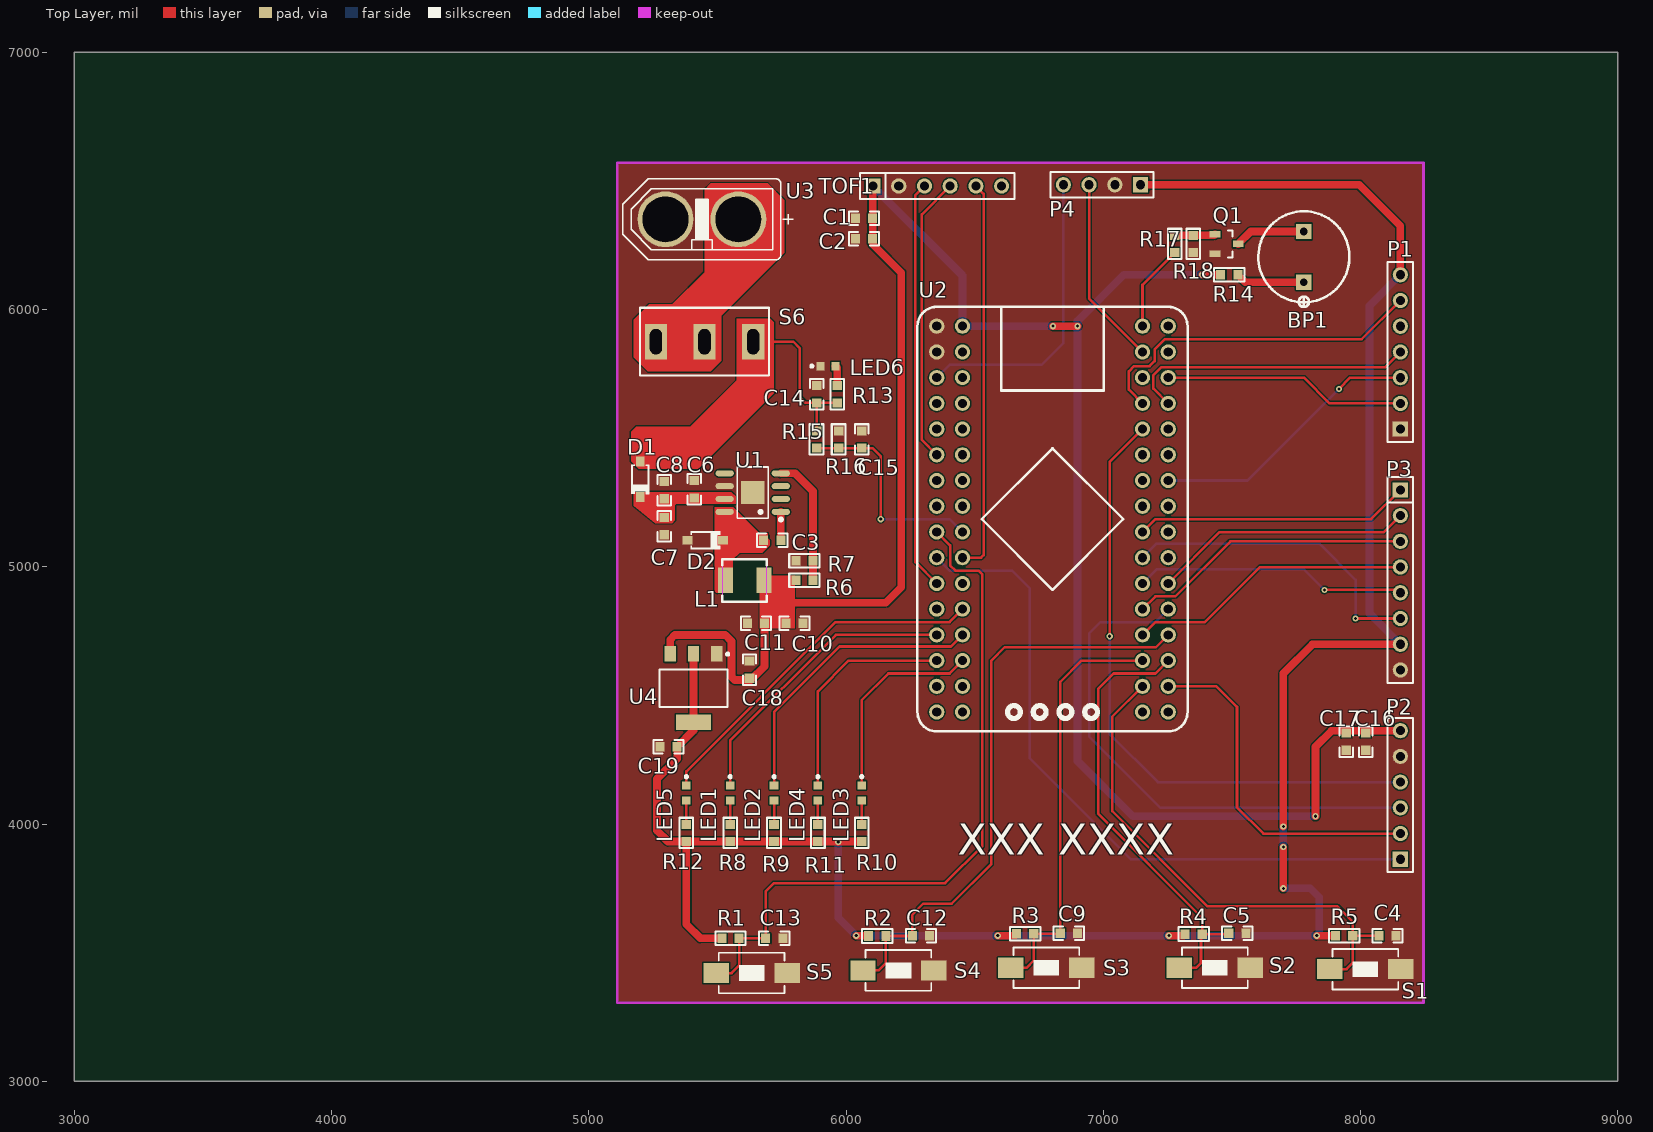
[diagram p0: Top Layer view]
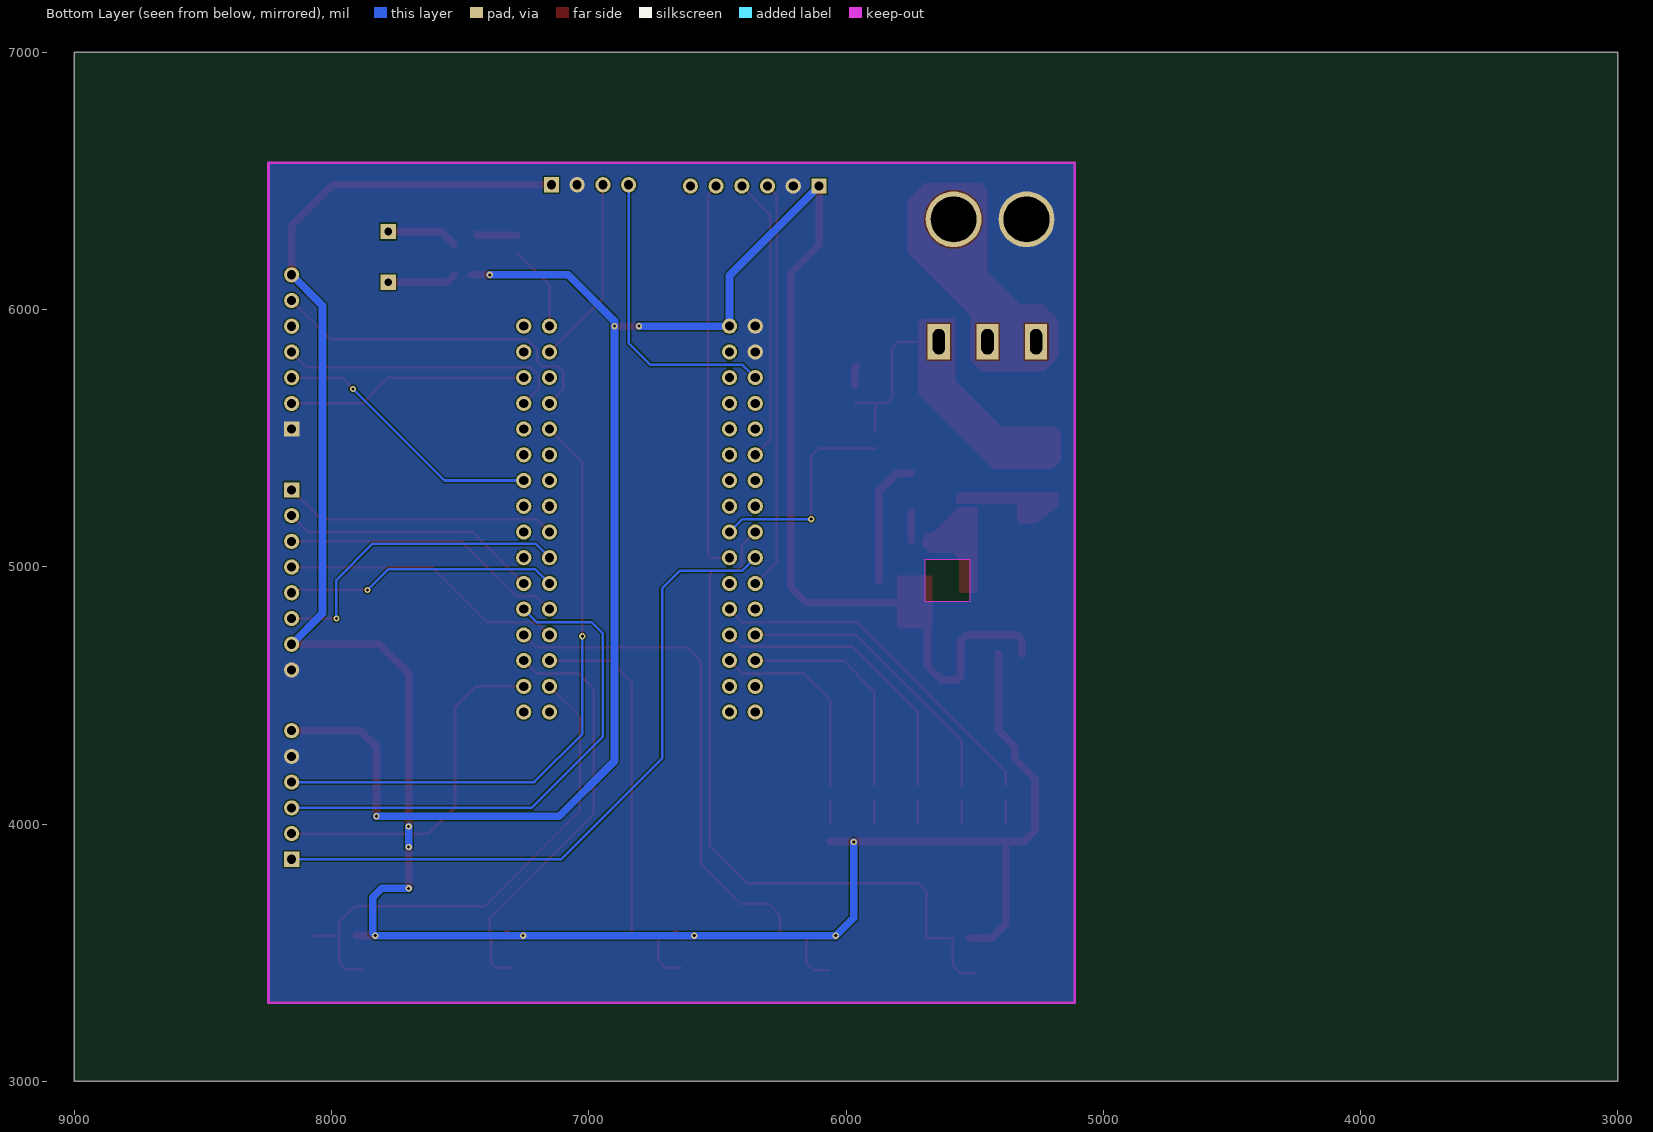
[diagram p1: Bottom Layer view, seen from below]
# Altium PCB MISC75116.pcbdoc
Units mil, origin at the board's own origin, x right, y up, seen from the top; angles counter-clockwise.
Board outline 6000 x 4000 mil, 2 copper layers (Top Layer, Bottom Layer); 63 components, 49 nets, 220 pads, 17 vias.

## Layer stack, top to bottom (the 12.6 mil dielectric is the usual default, probably not edited)
Top Solder Mask Layer: solder mask 0.4, Solder Resist, Dk 3.5
Top Layer: signal copper 1.4
Dielectric 1: surface 12.6, FR-4, Dk 4.8
Bottom Layer: signal copper 1.4
Bottom Solder Mask Layer: solder mask 0.4, Solder Resist, Dk 3.5

## Board outline
3000,7000 3000,3000 9000,3000 9000,7000

## Design rules (kind name [scope] priority, off if disabled: settings)
BoardOutlineClearance Clearance_1 [All] p2: genericclearance=5 ignorepadtopadclearanceinfootprint=FALSE except(0: Arc-SplitContinuation Track-SplitContinuation SMDPad-SplitContinuation THPad-SplitContinuation Via-SplitContinuation Fill-SplitContinuation Region-SplitContinuation Poly-SplitContinuation Text-SplitContinuation Hole-SplitContinuation; 5: Arc-OutlineEdge Track-OutlineEdge SMDPad-OutlineEdge THPad-OutlineEdge Via-OutlineEdge Fill-OutlineEdge Region-OutlineEdge Poly-OutlineEdge Text-OutlineEdge Hole-OutlineEdge SMDPad-CutoutEdge THPad-CutoutEdge Poly-CutoutEdge; 6: Via-CutoutEdge Fill-CutoutEdge Region-CutoutEdge Text-CutoutEdge; 6.9: Hole-CutoutEdge; 11.8: Arc-CutoutEdge Track-CutoutEdge)
Clearance [All] p1: gap=5 ignorepadtopadclearanceinfootprint=FALSE
DiffPairsRouting [All] p1: maxlimit=10 minlimit=6 mostfreqgap=6 toplayer_minwidth=15 toplayer_prefwidth=15 toplayer_maxwidth=15 toplayer_mingap=10 toplayer_prefgap=10 toplayer_maxgap=10 bottomlayer_minwidth=15 bottomlayer_prefwidth=15 bottomlayer_maxwidth=15 bottomlayer_mingap=10 bottomlayer_prefgap=10 bottomlayer_maxgap=10 maxuncoupledlength=10
HoleToHoleClearance ComponentClearance [All] p1: gap=10 allowstackedmicrovias=TRUE
Length netLength [All] p1: minlimit=0 maxlimit=0
MatchedLengths netLengthTolerance [All] p1: tolerance=1000
PlaneConnect [All] p1: planeconnectstyle=Direct reliefexpansion=20 reliefentries=4 reliefconductorwidth=10 reliefairgap=10
PolygonConnect [(InNet('GND'))] p1: connectstyle=Direct reliefconductorwidth=10 reliefentries=4 polygonreliefangle="90 Angle" airgapwidth=10 via.connectstyle=Relief via.reliefconductorwidth=10 via.reliefentries=4 via.polygonreliefangle="90 Angle" via.airgapwidth=10
RoutingVias [All] p1: holewidth=28 width=50 viastyle="Through Hole" minholewidth=2 minwidth=2 maxholewidth=28 maxwidth=50
SolderMaskExpansion [All] p1: expansion=4 istentingtop=FALSE
Width [All] p1: maxlimit=10 minlimit=10 preferedwidth=10 toplayer_minwidth=10 toplayer_maxwidth=200 toplayer_prefwidth=10 bottomlayer_minwidth=10 bottomlayer_maxwidth=200 bottomlayer_prefwidth=10
1 further rules are at their usual default settings.

## Components (designator, comment, footprint, x,y, rotation, side; value= is the part's Value field where it differs from the comment)
BP1 "Buzzer" 5*10fengmiqi 7780,6205 r90 top
C1 "10uF" CAPC1608[0603]S-N 6070.16,6354.81 r0 top
C2 "0.1uF" CAPC1608[0603]S-N 6070.16,6275.25 r0 top
C3 "100nF" CAPC1608[0603]S-N 5713.43,5103.06 r180 top
C4 "10uF" CAPC1608[0603]S-N 8105,3565 r0 top
C5 "10uF" CAPC1608[0603]S-N 7521.45,3575.86 r0 top
C6 "0.1uF" CAPC1608[0603]S-N 5409.96,5301.52 r270 top
C7 "4.7uF" CAPC1608[0603]S-N 5293.43,5158.06 r90 top
C8 "4.7uF" CAPC1608[0603]S-N 5293.43,5298.06 r270 top
C9 "10uF" CAPC1608[0603]S-N 6866.45,3575.86 r0 top
C10 "100uF" CAPC1608[0603]S-N 5800,4780 r0 top
C11 "0.1uF" CAPC1608[0603]S-N 5650,4780 r0 top
C12 "10uF" CAPC1608[0603]S-N 6291.45,3565.86 r0 top
C13 "10uF" CAPC1608[0603]S-N 5721.16,3555.57 r0 top
C14 "1000uF  25V" CAPC1608[0603]S-N 5885.73,5670.69 r90 top
C15 "100nF 50V X7R" CAPC1608[0603]S-N 6060.57,5495 r90 top
C16 "0.1uF ±10% 25V" CAPC1608[0603]S-N 8020,4320 r270 top
C17 "10uF ±10% 50V" CAPC1608[0603]S-N 7945,4320 r270 top
C18 "1uF" CAPC1608[0603]S-N 5625,4600 r270 top
C19 "1uF" CAPC1608[0603]S-N 5310,4300 r0 top
D1 "SS54" SOD-123-L 5200,5340 r270 top
D2 "SS54" SOD-123-L 5453.43,5103.06 r0 top
L1 "4.7uH 2.5A" "0402 TPC 4*4*2" 5573.43,4893.06 r270 top
LED1 "LED" LEDC1608(0603) 5549.84,4120.74 r270 top
LED2 "LED" LEDC1608(0603) 5720.31,4120.74 r270 top
LED3 "LED" LEDC1608(0603) 6061.24,4120.74 r270 top
LED4 "LED" LEDC1608(0603) 5890.77,4120.74 r270 top
LED5 "LED" LEDC1608(0603) 5379.37,4120.74 r270 top
LED6 "LED" LEDC1608(0603) 5930,5780 r0 top
P1 "Header 7" HDR1X7 8155,5535 r90 top
P2 "Gyroscope" HDR1X6 8155,3862.78 r90 top
P3 "Header  1X8" HDR1X8 8155,5298.89 r270 top
P4 "Header-D-M 1x4P" HDR1X4 7145,6485 r180 top
Q1 "S8050" SOT-23 7479.78,6255.03 r0 top
R1 "1K" RESC1608[0603]S-N 5551.16,3555.57 r180 top
R2 "1K" RESC1608[0603]S-N 6121.45,3564.61 r180 top
R3 "1K" RESC1608[0603]S-N 6696.45,3573.36 r180 top
R4 "1K" RESC1608[0603]S-N 7351.45,3572.11 r180 top
R5 "1K" RESC1608[0603]S-N 7936.45,3565.86 r180 top
R6 "10K" RESC1608[0603]S-N 5838.43,4948.06 r180 top
R7 "3K" RESC1608[0603]S-N 5838.43,5023.06 r180 top
R8 "10K" RESC1608[0603]S-N 5549.84,3965.27 r90 top
R9 "10K" RESC1608[0603]S-N 5720.31,3965.27 r90 top
R10 "10K" RESC1608[0603]S-N 6061.24,3965.27 r90 top
R11 "10K" RESC1608[0603]S-N 5890.77,3965.27 r90 top
R12 "10K" RESC1608[0603]S-N 5379.37,3965.27 r90 top
R13 "1K" RESC1608[0603]S-N 5965.87,5670.69 r90 top
R14 "10R ±1%" RESC1608[0603]S-N 7490,6135 r0 top
R15 "10K ±1%" RESC1608[0603]S-N 5885.57,5495 r270 top
R16 "1K ±1%" RESC1608[0603]S-N 5971.15,5495 r90 top
R17 "4.7K ±1%" RESC1608[0603]S-N 7278.09,6255.03 r90 top
R18 "10K ±1%" RESC1608[0603]S-N 7350,6255 r270 top
S1 "KEY" anjiantiepiankaiguan 8021.45,3435.86 r0 top
S2 "KEY" anjiantiepiankaiguan 7436.45,3440.86 r0 top
S3 "KEY" anjiantiepiankaiguan 6781.45,3440.86 r0 top
S4 "KEY" anjiantiepiankaiguan 6206.45,3430.86 r0 top
S5 "KEY" anjiantiepiankaiguan 5636.16,3420.57 r0 top
S6 "SW" SS12D10 5450,5875 r0 top
TOF1 "Ranging module" HDR1X6 6105,6480 r0 top
U1 "TPS5450" 5450 5603.43,5283.06 r90 top
U2 "STC32G12K128" STC16F40K128_CoreBoard 6802.78,5185.25 r0 top
U3 "XT60-F" XT60 5455.61,6421.45 r0 top
U4 "LM1117" "LM1117 - duplicate" 5417.17,4518.45 r180 top

## Footprints (in the part's own frame and the unit in brackets; to place one, negate y for a bottom-side part, rotate by r counter-clockwise, add the part's x,y. Pads: shape width x height; smd on the part's side, far side on the other; paste and mask are expansions set on the pad)
5*10fengmiqi [mil]
  rect 60x60 hole 30: 1(-98.43,0) 2(98.43,0)
  silkscreen extent -195,-177 177,177
"0402 TPC 4*4*2" [mm]
  rect 2.5x1.5 smd: 1(-1.371,-1.076) 2(-1.371,2.724)
  silkscreen extent -3.47,-1.38 0.73,3.02
5450 [mm]
  oval 0.6x1.8 smd paste+0 mask+0.051: 1(-1.77,-3.638) 2(-0.5,-3.638) 3(0.77,-3.638) 4(2.04,-3.638) 5(2.04,1.907) 6(0.77,1.907) 7(-0.5,1.907) 8(-1.77,1.907)
  rect 2.29x2.29 smd paste+0 mask+0.051: 9(0.135,-0.866)
  silkscreen extent -2.67,-3.79 2.66,0.66
anjiantiepiankaiguan [mm]
  rect 2.5x2 smd: 1(3.429,0) 2(-3.571,0)
  silkscreen extent -3.32,-2 3.18,2
CAPC1608[0603]S-N [mm]
  rect 0.9x0.95 smd: 1(-0.85,0) 2(0.85,0)
  silkscreen extent -1.5,-0.66 1.5,0.66
HDR1X4 [mm]
  rect 1.5x1.5 hole 0.9: 1(0,0)
  round 1.5 hole 0.9: 2(2.54,0) 3(5.08,0) 4(7.62,0)
  silkscreen extent -1.27,-1.27 8.89,1.27
HDR1X6 [mm]
  rect 1.5x1.5 hole 0.9: 1(0,0)
  round 1.5 hole 0.9: 2(2.54,0) 3(5.08,0) 4(7.62,0) 5(10.16,0) 6(12.7,0)
  silkscreen extent -1.27,-1.27 13.97,1.27
HDR1X7 [mm]
  rect 1.5x1.5 hole 0.9: 1(0,0)
  round 1.5 hole 0.9: 2(2.54,0) 3(5.08,0) 4(7.62,0) 5(10.16,0) 6(12.7,0) 7(15.24,0)
  silkscreen extent -1.27,-1.27 16.51,1.27
HDR1X8 [mm]
  rect 1.5x1.5 hole 0.9: 1(0,0)
  round 1.5 hole 0.9: 2(2.54,0) 3(5.08,0) 4(7.62,0) 5(10.16,0) 6(12.7,0) 7(15.24,0) 8(17.78,0)
  silkscreen extent -1.27,-1.27 19.05,1.27
LEDC1608(0603) [mm]
  rect 0.8x0.85 smd: A(0.75,0) C(-0.75,0)
  silkscreen extent -1.72,-0.12 -1.48,0.12
"LM1117 - duplicate" [mm]
  rect 1.1x1.55 smd: 1(-2.046,-3.629) 2(0.254,-3.629) 3(2.554,-3.629)
  rect 3.45x1.55 smd: 4(0.254,3.121)
  silkscreen extent -3.25,-3.73 3.6,1.6
RESC1608[0603]S-N [mm]
  rect 0.9x0.95 smd: 1(-0.85,0) 2(0.85,0)
  silkscreen extent -1.5,-0.67 1.5,0.67
SOD-123-L [mm]
  rect 1x0.85 smd: A(-1.75,0) K(1.75,0)
  silkscreen extent -1.45,-0.9 1.47,0.9
SOT-23 [mm]
  rect 1.05x0.65 smd: 1(-1.15,0.95) 2(-1.15,-0.95) 3(1.15,0)
  silkscreen extent 0.13,-1.35 0.58,1.35
SS12D10 [mm]
  rect 2.2x3.5 hole 1.2 slot 2.5 at 90 deg paste+0 mask+0.07: 1(-4.8,0) 2(0,0) 3(4.8,0)
  silkscreen extent -6.35,-3.35 6.35,3.35
STC16F40K128_CoreBoard [mm]
  round 1.5 hole 0.9: 1(-11.43,19.05) 2(-8.89,19.05) 3(-11.43,16.51) 4(-8.89,16.51) 5(-11.43,13.97) 6(-8.89,13.97) 7(-11.43,11.43) 8(-8.89,11.43) 9(-11.43,8.89) 10(-8.89,8.89) 11(-11.43,6.35) 12(-8.89,6.35) 13(-11.43,3.81) 14(-8.89,3.81) 15(-11.43,1.27) 16(-8.89,1.27) 17(-11.43,-1.27) 18(-8.89,-1.27) 19(-11.43,-3.81) 20(-8.89,-3.81) 21(-11.43,-6.35) 22(-8.89,-6.35) 23(-11.43,-8.89) 24(-8.89,-8.89) 25(-11.43,-11.43) 26(-8.89,-11.43) 27(-11.43,-13.97) 28(-8.89,-13.97) 29(-11.43,-16.51) 30(-8.89,-16.51) 31(-11.43,-19.05) 32(-8.89,-19.05) 33(8.89,-19.05) 34(11.43,-19.05) 35(8.89,-16.51) 36(11.43,-16.51) 37(8.89,-13.97) 38(11.43,-13.97) 39(8.89,-11.43) 40(11.43,-11.43) 41(8.89,-8.89) 42(11.43,-8.89) 43(8.89,-6.35) 44(11.43,-6.35) 45(8.89,-3.81) 46(11.43,-3.81) 47(8.89,-1.27) 48(11.43,-1.27) 49(8.89,1.27) 50(11.43,1.27) 51(8.89,3.81) 52(11.43,3.81) 53(8.89,6.35) 54(11.43,6.35) 55(8.89,8.89) 56(11.43,8.89) 57(8.89,11.43) 58(11.43,11.43) 59(8.89,13.97) 60(11.43,13.97) 61(8.89,16.51) 62(11.43,16.51) 63(8.89,19.05) 64(11.43,19.05)
  silkscreen extent -13.33,-20.95 13.33,20.95
XT60 [mil]
  round 217.16 hole 177.16 slot 177.36 at 0 deg paste+0 mask+2: ""(-157.43,-70.62) ""(126.03,-70.62)
  silkscreen extent -323,-228 339,87

## Via types
v1: diameter 24.02, hole 12, Top Layer to Bottom Layer, 17 vias

## Nets (pads, with @x,y where several pads share a name; then routed paths per layer and width w, separated by ;. In a path a pad name is that pad's centre, name@x,y a point inside that pad or via, vN(x,y) a via of type N, cw(c..) or ccw(c..) an arc to the next point about the centre after c; other vN are vias at no path point)
0.2: P1.3 U2.52 | length 1067.8
  Top Layer w10: v1(7916.35,5691.35) 7960,5735 P1.3
  Bottom Layer w10: U2.52 7560.25,5335.25 v1(7916.35,5691.35)
0.3: P1.4 U2.58 | length 1131
  Top Layer w10: U2.58 7195,5693.03 7195,5745 7225,5775 8095,5775 P1.4
1.0: P4.3 U2.61 | length 735.8
  Top Layer w10: P4.3 6945,6043.03 U2.61
1.1: P4.4 U2.5 | length 1163
  Bottom Layer w10: U2.5 6402.53,5785 6760,5785 6845,5870 P4.4
3V3: C19.2 P1.7 P3.7 P4.1 R1.2 R2.2 R3.2 R4.2 R5.2 R8.1 R9.1 R10.1 R11.1 R12.1 U4.2 U4.4 | length 8936.2
  Top Layer w30: U4.2 U4.4 5407.17,4363.71 C19.2 5343.46,4253.46 5265,4175 5265,3975 5308.19,3931.81 R12.1 ; R1.2 5434.43,3555.57 5379.37,3610.63 R12.1 ; v1(6040,3565.86) 6086.73,3565.86 R2.2 ; R10.1 5971.81,3931.81 v1(5970,3930) 5968.19,3931.81 R11.1 R9.1 R8.1 R12.1 ; v1(6590,3565.86) 6655.48,3565.86 R3.2 ; P4.1 7995,6485 8155,6325 P1.7 ; v1(7255,3565.86) 7311.73,3565.86 R4.2 ; v1(7700,3750) v1(7700,3910) ; v1(7700,3990) 7700,4585 7813.89,4698.89 P3.7 ; v1(7830,3565.86) R5.2
  Bottom Layer w30: v1(5970,3930) 5970,3635.86 v1(6040,3565.86) v1(6590,3565.86) v1(7255,3565.86) v1(7830,3565.86) 7840,3575.86 7840,3715 7805,3750 v1(7700,3750) ; v1(7700,3910) v1(7700,3990) ; P3.7 8035,4818.89 8035,6015 P1.7
4: P1.6 U2.57 | length 1342.3
  Top Layer w10: U2.57 7099.52,5688.51 7099.52,5759.52 7120,5780 7180,5780 7200,5800 7200,5845 7240,5885 8005,5885 P1.6
5: P1.2 U2.60 | length 943.7
  Top Layer w10: U2.60 7779.75,5735.25 7880,5635 P1.2
5V: C1.2 C2.2 C10.1 C11.2 C16.1 C17.1 C18.2 L1.2 P2.6 R6.2 R14.1 TOF1.1 U2.2 U4.3 | length 7965.5
  Top Layer w30: U4.3 5316.62,4716.62 5335,4735 5530,4735 5555,4710 5555,4572.08 5567.08,4560 5630,4560 5683.46,4613.46 C11.2 ; 5770,4860 6155,4860 6215,4920 6215,6142.84 6103.62,6254.21 C2.2 C1.2 6103.62,6478.62 TOF1.1 ; v1(6805,5935.25) v1(6900,5935.25) ; v1(7385,6135) R14.1 ; v1(7825,4030) 7825,4300 7887.78,4362.78 P2.6
  Bottom Layer w30: TOF1.1 6452.78,6132.22 U2.2 v1(6805,5935.25) ; v1(7385,6135) 7080,6135 6900,5955 v1(6900,5935.25) 6900,4245 7115,4030 v1(7825,4030)
12V: C14.1 D1.A R13.1 R15.1 S6.3 | length 645.5
  Top Layer w10: S6.3 5795,5875 5820,5850 5820,5660 5842.78,5637.22 C14.1 ; R15.1 5885.73,5528.62 C14.1 ; R13.1 C14.1
17: C15.1 R15.2 R16.1 U2.18 | length 845.9
  Top Layer w10: R15.2 R16.1 C15.1 6103.46,5461.54 6135,5430 v1(6135,5185)
  Bottom Layer w10: v1(6135,5185) 6403.03,5185 U2.18
20: P3.4 U2.39 | length 1111.4
  Top Layer w10: U2.39 7202.53,4785 7395,4785 7608.89,4998.89 P3.4
21: P3.3 U2.41 | length 1111.4
  Top Layer w10: U2.41 7202.53,4885 7280,4885 7493.89,5098.89 P3.3
22: P3.2 U2.44 | length 1011.4
  Top Layer w10: U2.44 7452.53,5135 8091.11,5135 P3.2
23: P3.5 U2.43 | length 1062.6
  Top Layer w10: v1(7860,4910) 8143.89,4910 P3.5
  Bottom Layer w10: U2.43 7207.53,4990 7780,4990 v1(7860,4910)
25: P3.6 U2.45 | length 1233.3
  Top Layer w10: v1(7981.11,4798.89) P3.6
  Bottom Layer w10: U2.45 7207.53,5090 7840,5090 7981.11,4948.89 v1(7981.11,4798.89)
27: P3.1 U2.47 | length 1070
  Top Layer w10: U2.47 7202.53,5185 8041.11,5185 P3.1
30: LED1.C U2.25 | length 1147.5
  Top Layer w10: LED1.C 5549.84,4324.84 5960.25,4735.25 U2.25
31: LED2.C U2.26 | length 1141.8
  Top Layer w10: LED2.C 5720.31,4435.31 5975,4690 6407.53,4690 U2.26
32: LED3.C U2.28 | length 786.3
  Top Layer w10: LED3.C 6061.24,4481.24 6165,4585 6402.53,4585 U2.28
33: LED4.C U2.27 | length 877
  Top Layer w10: LED4.C 5890.77,4515.77 6010.25,4635.25 U2.27
40: P2.1 U2.19 | length 2674.5
  Bottom Layer w10: U2.19 6403.03,4985 6645,4985 6715,4915 6715,4255 7107.22,3862.78 P2.1
41: P2.2 U2.36 | length 1367.8
  Top Layer w10: U2.36 7439.75,4535.25 7520,4455 7520,4065 7622.22,3962.78 P2.2
42: P2.3 U2.42 | length 2072.1
  Bottom Layer w10: U2.42 7202.53,4785 6990,4785 6945,4740 6945,4340 7222.22,4062.78 P2.3
43: P2.4 U2.55 | length 2445.7
  Top Layer w10: v1(7025,4730) 7025,5407.47 U2.55
  Bottom Layer w10: v1(7025,4730) 7025,4350 7212.22,4162.78 P2.4
46: R17.1 U2.63 | length 338.2
  Top Layer w10: U2.63 7152.78,6096.25 R17.1
47: TOF1.5 U2.20 | length 1533.7
  Top Layer w10: U2.20 6525.25,5035.25 6535,5045 6535,6450 TOF1.5
63: TOF1.4 U2.11 | length 1114.2
  Top Layer w10: U2.11 6295,5493.03 6295,6370 TOF1.4
65: TOF1.3 U2.21 | length 1593.5
  Top Layer w10: TOF1.3 6270,6445 6270,5018.03 U2.21
66: LED5.C U2.24 | length 1388.8
  Top Layer w10: LED5.C 5379.37,4204.37 5960,4785 6402.53,4785 U2.24
70: C4.1 R5.1 S1.2 U2.35 | length 2008.2
  Top Layer w10: U2.35 7035,4417.47 7035,4050 7405,3680 7910,3680 7969.91,3620.09 R5.1 ; S1.2 7945.86,3435.86 7969.91,3459.91 R5.1 ; C4.1 8070.68,3565.86 R5.1
71: C5.1 R4.1 S2.2 U2.38 | length 1749.9
  Top Layer w10: U2.38 7202.53,4585 7040,4585 6980,4525 6980,4040 7384.91,3635.09 R4.1 ; S2.2 7360.86,3440.86 7380,3460 7380,3567.2 R4.1 ; C5.1 7484.23,3572.11 R4.1
72: C9.1 R3.1 S3.2 U2.37 | length 1639.6
  Top Layer w10: S3.2 6700.86,3440.86 6729.91,3469.91 R3.1 6830.48,3573.36 C9.1 6832.98,4552.98 6915.25,4635.25 U2.37
73: C12.1 R2.1 S4.2 U2.40 | length 2299.4
  Top Layer w10: S4.2 6125.86,3430.86 6154.91,3459.91 R2.1 6256.73,3564.61 C12.1 6257.98,3647.98 6300,3690 6410,3690 6565,3845 6565,4635 6617.07,4687.07 7204.6,4687.07 U2.40
GND: C1.1 C2.1 C4.2 C5.2 C6.1 C7.1 C8.1 C9.2 C10.2 C11.1 C12.2 C13.2 C14.2 C15.2 C16.2 C17.2 C18.1 C19.1 D2.A LED6.C P1.1 P2.5 P3.8 P4.2 Q1.2 R7.2 R16.2 R18.2 S1.1 S2.1 S3.1 S4.1 S5.1 TOF1.2 U1.6 U1.9 U2.1 U2.3 U3.@5298.18,6350.83 U4.1
NetBP1_1: BP1.1 R14.2 | length 268.3
  Top Layer w30: R14.2 7551.89,6106.57 BP1.1
NetBP1_2: BP1.2 Q1.3 | length 275
  Top Layer w30: Q1.3 7573.46,6303.43 BP1.2
NetC3_1: C3.1 U1.1 | length 110.4
  Top Layer w30: U1.1 5746.67,5103.28 C3.1
NetC3_2: C3.2 D2.K L1.1 U1.8
NetC6_2: C6.2 C7.2 C8.2 D1.K U1.7
NetLED1_A: LED1.A R8.2 | length 92.5
  Top Layer w10: R8.2 LED1.A
NetLED2_A: LED2.A R9.2 | length 92.5
  Top Layer w10: R9.2 LED2.A
NetLED3_A: LED3.A R10.2 | length 92.5
  Top Layer w10: R10.2 LED3.A
NetLED4_A: LED4.A R11.2 | length 92.5
  Top Layer w10: R11.2 LED4.A
NetLED5_A: LED5.A R12.2 | length 92.5
  Top Layer w10: R12.2 LED5.A
NetLED6_A: LED6.A R13.2 | length 78.5
  Top Layer w30: LED6.A 5965.87,5773.66 R13.2
NetQ1_1: Q1.1 R17.2 R18.1 | length 158
  Top Layer w30: R17.2 R18.1 7430.57,6288.49 Q1.1
NetR6_1: R6.1 R7.1 U1.4 | length 499.4
  Top Layer w30: U1.4 5801.64,5363.36 5871.89,5293.11 R7.1 R6.1
NetS6_1: S6.1 S6.2 U3.@5581.64,6350.83
RST: C13.1 R1.1 S5.2 U2.17 | length 2754.4
  Top Layer w10: S5.2 5555.57,3420.57 5584.62,3449.62 R1.1 C13.1 5687.69,3737.69 5720,3770 6385,3770 6530,3915 6530,4970.11 6515.11,4985 6425,4985 6405,5005 6405,5083.03 U2.17
pads on no net: P1.5 TOF1.6 U1.2 U1.3 U1.5 U2.4 U2.6 U2.7 U2.8 U2.9 U2.10 U2.12 U2.13 U2.14 U2.15 U2.16 U2.22 U2.23 U2.29 U2.30 U2.31 U2.32 U2.33 U2.34 U2.46 U2.48 U2.49 U2.50 U2.51 U2.53 U2.54 U2.56 U2.59 U2.62 U2.64

## Polygon pours and split planes (outlines as drawn)
GND on Top Layer (solid, remove dead copper, pour order 0): 4945,6705 4945,3200 8495,3200 8495,6705
GND on Bottom Layer (solid, remove dead copper, pour order 2): 5015,6705 5015,3230 8480,3230 8480,6705

## Keep-outs
Board Outline Layer:
  region: 5519.26,5029.72 5519.26,4863.15 5692.49,4863.15 5692.49,5029.72
  lines w10: 5110,3305 5110,6570 8245,6570 8245,3305 5110,3305

## Other copper
Top Layer:
  region net NetS6_1: 5475,6490 5695,6490 5760,6425 5760,6220 5515,5975 5515,5800 5475,5760 5230,5760 5175,5815 5175,5960 5235,6020 5324.99,6020 5450.01,6145.02 5450.01,6465.01
  region net 12V: 5575,5965 5705,5965 5720,5950 5720,5675 5425.81,5380.81 5193.72,5380.81 5164.57,5409.97 5164.57,5524.57 5185,5545 5395,5545 5575,5725
  region net NetC3_2: 5561.64,5231.55 5663.2,5130 5695,5130 5695,5111.59 5703.53,5103.06 5703.53,5083.53 5675,5055 5586.15,5055 5559.76,5028.6 5559.76,4899.76 5495.24,4899.76 5490,4905 5490,5231.55
  region net 5V: 5665,4965 5665,4761.3 5800,4761.3 5800,4965
  region net NetC6_2: 5429.65,5290 5554.5,5290 5571.14,5273.36 5571.14,5245 5340,5245 5335,5240 5335,5180 5325,5170 5258.83,5170 5175,5237.97 5175,5285 5180,5290

## Silkscreen, mask and mechanical layers (free items; w line width, h text height)
Top Silkscreen Layer:
  text "XXX XXXX" at 6435,3880 h120